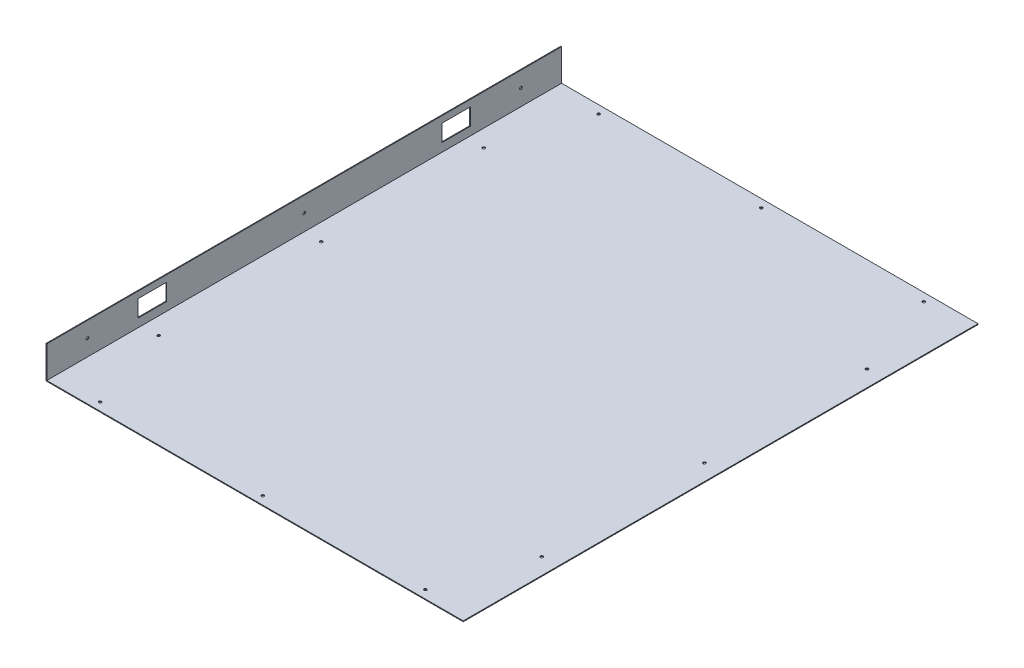
SolidWorks part; units mm, degrees
ref_plane "Front Plane" through (0, 0, 0) normal (0, 0, 1) x (1, 0, 0)
ref_plane "Top Plane" through (0, 0, 0) normal (0, 1, 0) x (1, 0, 0)
ref_plane "Right Plane" through (0, 0, 0) normal (1, 0, 0) x (0, 0, -1)
sketch "Sketch1" plane through (0, 0, 0) normal (0, 0, 1) x (1, 0, 0)
  line L0 (0, 0) -> (0, -60)
  line L1 (0, -60) -> (770, -60)
  line L2 (770, -60) -> (770, 0)
  line L3 (1.5, 0) -> (1.5, -58.5)
  line L4 (1.5, -58.5) -> (768.5, -58.5)
  line L5 (768.5, -58.5) -> (768.5, 0)
  line L6 (0, 0) -> (1.5, 0)
  line L7 (768.5, 0) -> (770, 0)
  dimension "D1" = 770
  dimension "D3" = 60
  dimension "D4" = 60
  dimension "D2" = 1.5
extrude "Boss-Extrude1" add sketch "Sketch1" along normal blind 950
sketch "Sketch2" plane through (770, 0, 0) normal (1, 0, 0) x (0, 0, -1)
  line L0 (0, -60) -> (0, 0) construction
  line L5 (-475, 0) -> (-475, 85.5947) construction
  line L6 (-729, -43) -> (-782, -12) construction
  line L7 (-221, -12) -> (-168, -12)
  line L8 (-221, -12) -> (-221, -43)
  line L9 (-221, -43) -> (-168, -43)
  line L10 (-168, -12) -> (-168, -43)
  line L11 (-221, -12) -> (-168, -43) construction
  line L12 (-221, -43) -> (-168, -12) construction
  line L13 (-950, 0) -> (0, 0) construction
  line L14 (-729, -12) -> (-782, -43) construction
  line L15 (-782, -12) -> (-782, -43)
  line L16 (-729, -43) -> (-782, -43)
  line L17 (-729, -12) -> (-729, -43)
  line L18 (-729, -12) -> (-782, -12)
  line L19 (-950, -60) -> (-950, 0) construction
  circle A0 centre (-75, -28.5) radius 2.5
  circle A1 centre (-475, -28.5) radius 2.5
  circle A2 centre (-875, -28.5) radius 2.5
  point P5 (-194.5, -27.5)
  point P15 (-755.5, -27.5)
  dimension "D7" = 5
  dimension "D9" = 5
  dimension "D1" = 53
  dimension "D2" = 31
  dimension "D3" = 168
  dimension "D4" = 12
  dimension "D5" = 28.5
  dimension "D6" = 75
  dimension "D8" = 75
extrude "Cut-Extrude1" cut sketch "Sketch2" against normal blind 1356.5
sketch "Sketch3" plane through (0, -60, 0) normal (0, -1, 0) x (1, 0, 0)
  line L0 (770, 950) -> (770, 0) construction
  line L1 (0, 950) -> (770, 950) construction
  line L2 (770, 475) -> (547.713, 475) construction
  line L3 (0, 950) -> (0, 0) construction
  circle A0 centre (740, 475) radius 2.5
  circle A1 centre (740, 775) radius 2.5
  circle A2 centre (740, 175) radius 2.5
  circle A3 centre (33, 775) radius 2.5
  circle A4 centre (33, 475) radius 2.5
  circle A5 centre (33, 175) radius 2.5
  circle A6 centre (385, 935) radius 2.5
  circle A7 centre (685, 935) radius 2.5
  circle A8 centre (85, 935) radius 2.5
  circle A9 centre (85, 15) radius 2.5
  circle A10 centre (685, 15) radius 2.5
  circle A11 centre (385, 15) radius 2.5
  point P9 (770, 475)
  point P25 (385, 950)
  dimension "D4" = 5
  dimension "D9" = 5
  dimension "D1" = 300
  dimension "D2" = 300
  dimension "D3" = 33
  dimension "D6" = 15
  dimension "D7" = 300
  dimension "D8" = 300
  dimension "D5" = 2
extrude "Cut-Extrude2" cut sketch "Sketch3" against normal blind 1.5
sketch "Sketch5" plane through (0, 0, 0) normal (0, 1, 0) x (1, 0, 0)
  line L4 (770, 0) -> (768.5, 0)
  line L5 (768.5, 0) -> (768.5, -950)
  line L6 (768.5, -950) -> (770, -950)
  line L7 (770, -950) -> (770, 0)
  line L8 (770, 0) -> (768.5, 0)
  line L9 (768.5, 0) -> (768.5, -950)
  line L10 (768.5, -950) -> (770, -950)
  line L11 (770, -950) -> (770, 0)
  dimension "D1" = 0
extrude "Cut-Extrude4" cut sketch "Sketch5" against normal up to surface (58.5 mm away) up to face at (85, -58.5, 17.5)
